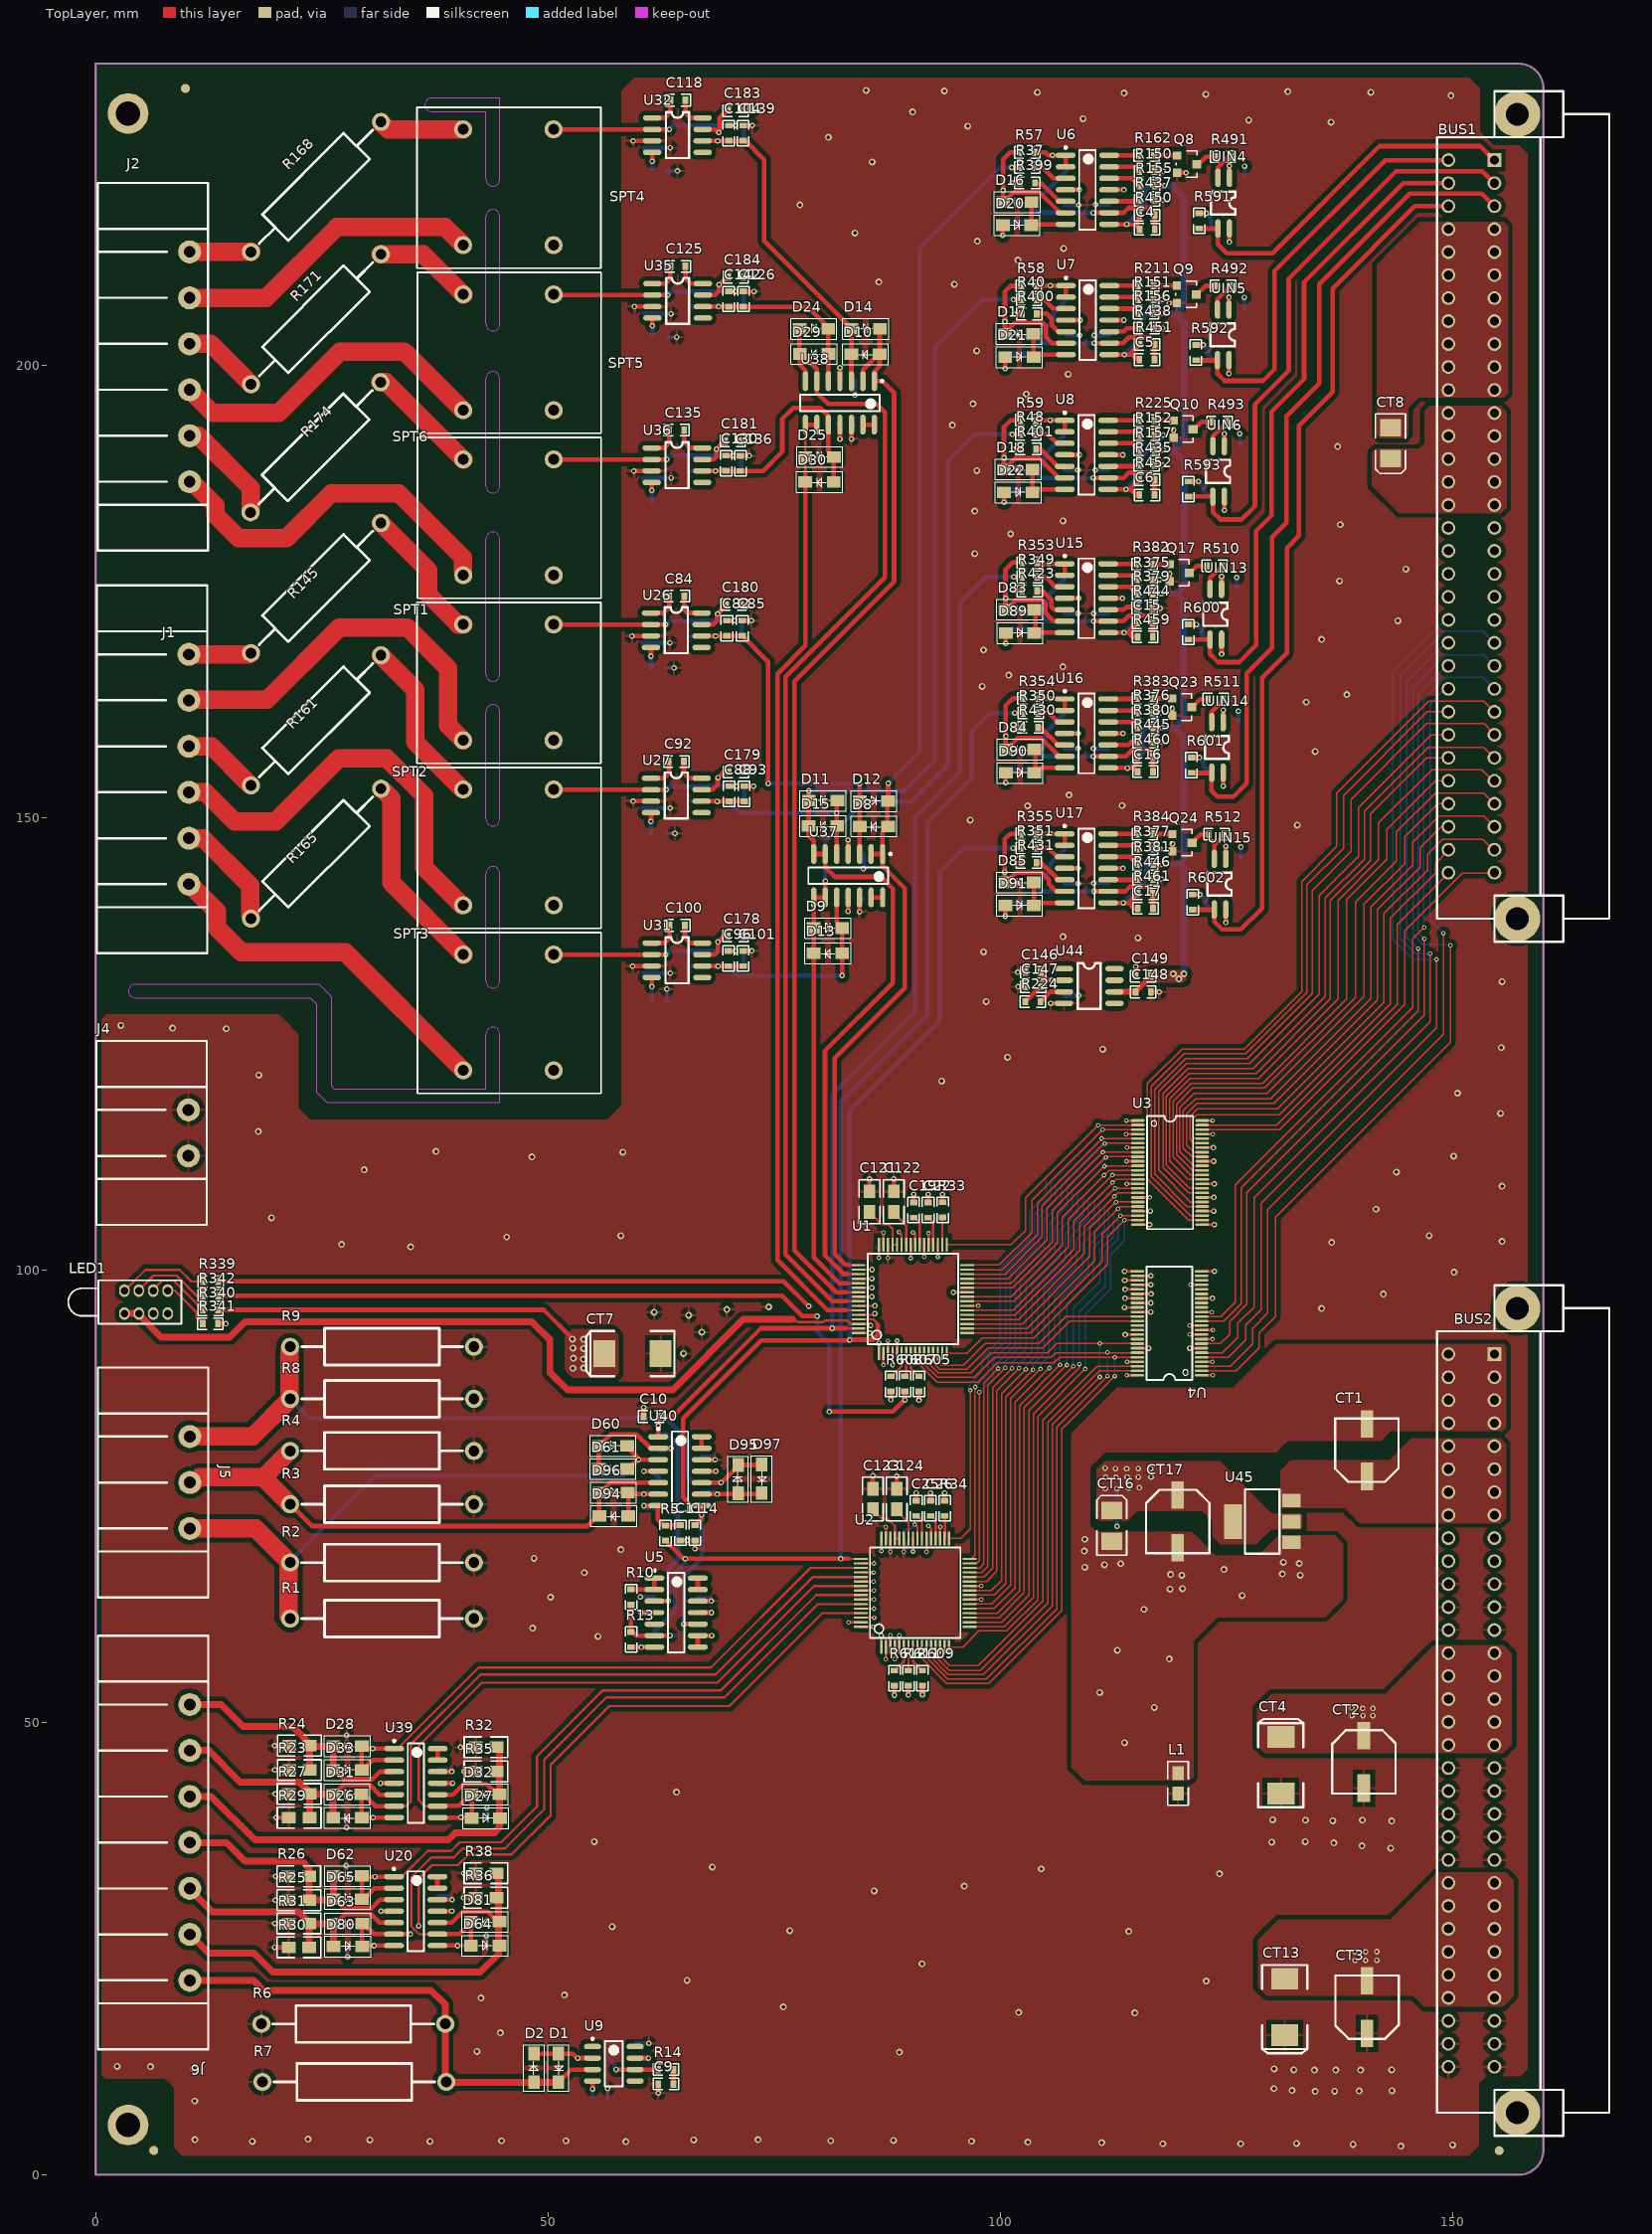
[diagram p0: TopLayer view]
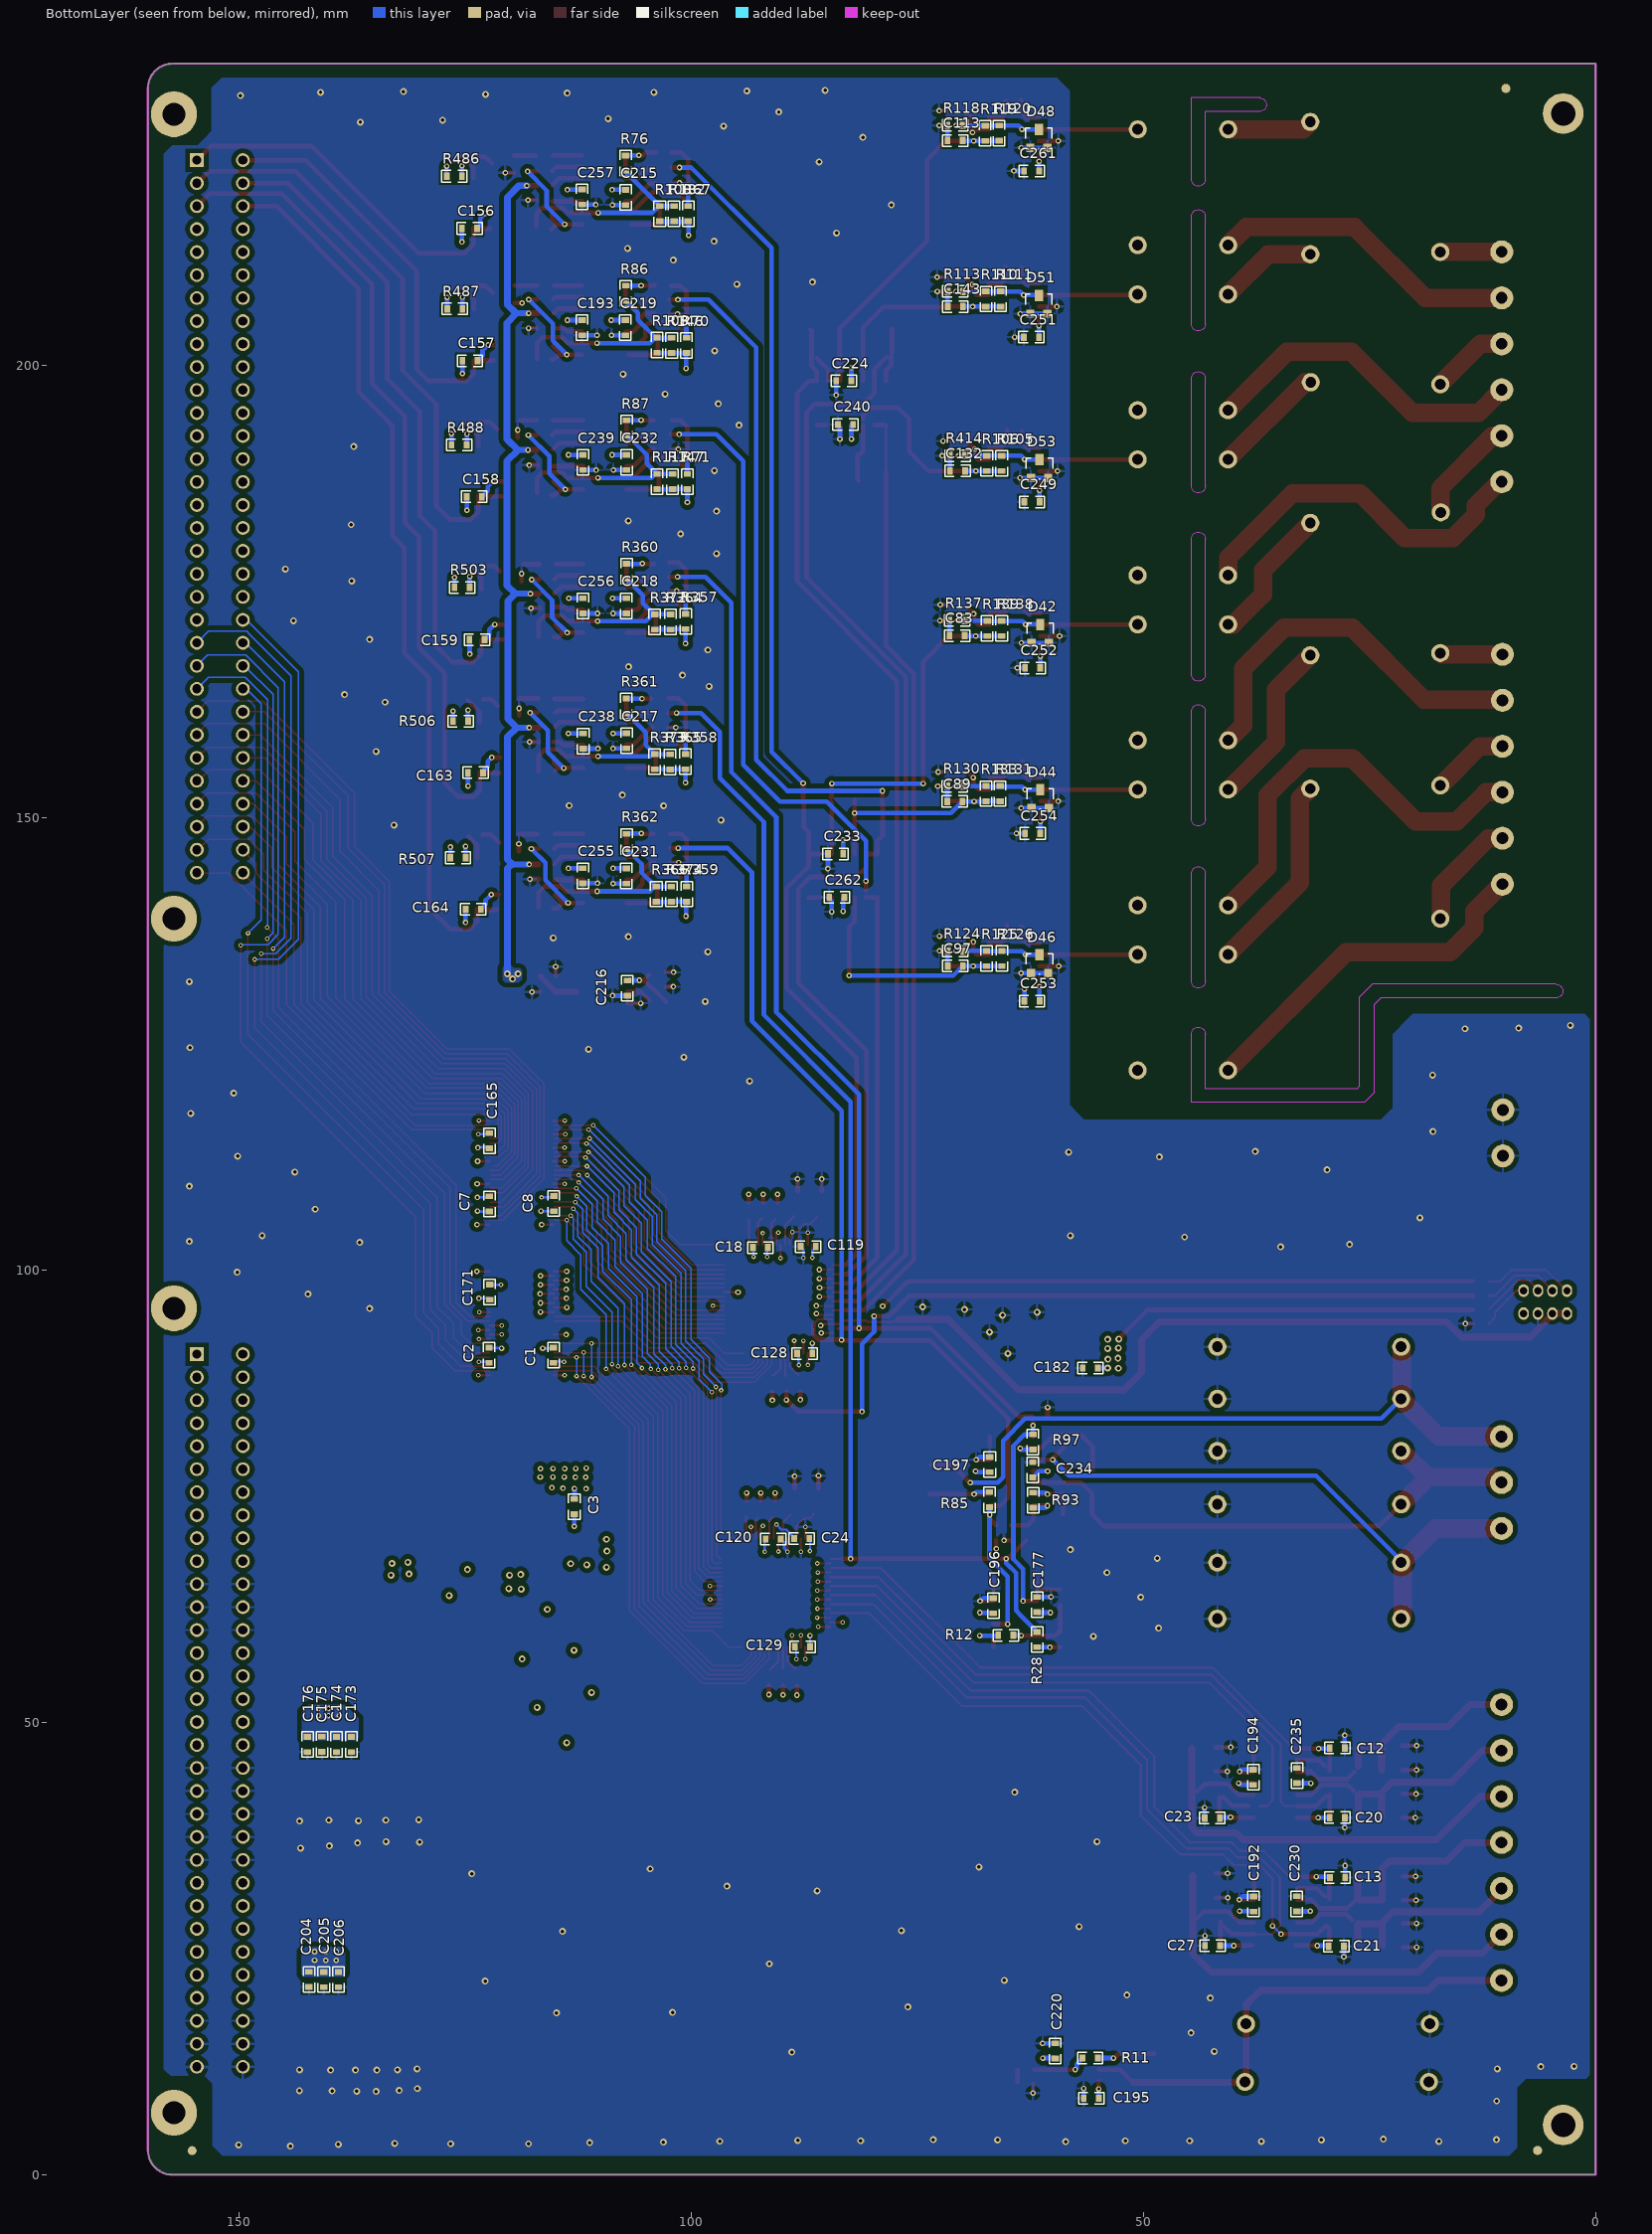
[diagram p1: BottomLayer view, seen from below]
# Altium PCB MISC80584.PCBDoc (part 1 of 7)
Units mm, origin at the board's own origin, x right, y up, seen from the top; angles counter-clockwise.
Board outline 160.02 x 233.3 mm, 4 copper layers (TopLayer, GND, POWER, BottomLayer); 386 components, 266 nets, 1374 pads, 640 vias.

## Layer stack, top to bottom (the 12.6 mil dielectric is the usual default, probably not edited)
TopLayer: signal copper 0.0356
Dielectric: core 0.32, FR-4, Dk 4.8
GND: plane copper 0.0356, net AGND
Dielectric: prepreg 0.32, FR-4, Dk 4.8
POWER: plane copper 0.0356, net (Multiple Nets)
Dielectric: core 0.32, FR-4, Dk 4.8
BottomLayer: signal copper 0.0356

## Board outline
0,0.025 0,233.324 157.302,233.324 cw(c157.302,230.607) 160.02,230.607 160.02,2.743 cw(c157.302,2.743) 157.302,0.025

## Design rules (kind name [scope] priority, off if disabled: settings)
Clearance Clearance_1 [inpolygon{AGND}] p1: gap=0.508
Clearance [All] p2: gap=0.14
FabricationTestPointUsage TestPointUsage [All] p1: valid=0 allowmultiple=FALSE
FabricationTestpoint Testpoint [(IsPad And (OnTopLayer Or OnBottomLayer))] p1: side=3 testpointundercomponent=TRUE minsize=1.016 maxsize=2.54 preferedsize=1.524 minholesize=0.508 maxholesize=1.016 preferedholesize=0.813 testpointgrid=0.025 allowsidetop=TRUE allowsidebottom=TRUE usegrid=TRUE gridtolerance=0
HoleSize [All] p1: absolutevalues=TRUE maxlimit=25.4 minlimit=0.025 maxpercent=80.000 minpercent=20.000
HoleToHoleClearance [All] p1: gap=0 allowstackedmicrovias=TRUE
MinimumSolderMaskSliver [All] p1: minsoldermaskwidth=0
PlaneClearance [All] p1: clearance=0.508
PlaneConnect [All] p1: planeconnectstyle=Direct reliefexpansion=0.508 reliefentries=4 reliefconductorwidth=0.254 reliefairgap=0.254
PolygonConnect PolygonConnect_1 [InNet(AGND)] p1: connectstyle=Relief reliefconductorwidth=0.305 reliefentries=4 polygonreliefangle="90 Angle"
PolygonConnect [All] p2: connectstyle=Direct reliefconductorwidth=0.254 reliefentries=4 polygonreliefangle="90 Angle"
RoutingVias [All] p1: holewidth=0.254 width=0.508 viastyle="Through Hole" minholewidth=0.254 minwidth=0.508 maxholewidth=0.305 maxwidth=0.61
SilkToSilkClearance [All] p1: silktosilkclearance=0
SilkscreenOverComponentPads [All] p1: minsilkscreentomaskgap=0
SolderMaskExpansion [All] p1: expansion=0.102
Width [All] p1: maxlimit=2.54 minlimit=0.152 preferedwidth=0.152 minimp=50.000000 maximp=50.000000 favimp=50.000000
19 further rules are at their usual default settings.

## Components (designator, comment, footprint, x,y, rotation, side; value= is the part's Value field where it differs from the comment)
BUS1 "CON64" BUS64W-A 154.61,222.656 r270 top
BUS2 "CON64" BUS64W-A 154.61,90.703 r270 top
C1 "0.1uF" 0603 115.189,89.764 r90 bottom
C2 "0.1uF" 0603 122.326,91.44 r270 bottom
C3 "0.1uF" 0603 112.903,74.701 r270 bottom
C4 "0.1uF" 0603 115.392,215.011 r0 top
C5 "0.1uF" 0603 115.367,200.609 r0 top
C6 "0.1uF" 0603 115.367,185.649 r0 top
C7 "0.1uF" 0603 122.276,106.477 r90 bottom
C8 "0.1uF" 0603 115.164,108.179 r270 bottom
C9 "0.1uF" 0603 62.205,10.058 r0 top
C10 "30p" 0603 60.579,83.82 r0 top
C11 "30p" 0603 64.618,70.129 r90 top
C12 "30p" 0603 27.737,47.193 r0 bottom
C13 "30p" 0603 27.711,32.868 r0 bottom
C14 "30p" 0603 66.243,70.129 r90 top
C15 "0.1uF" 0603 115.138,171.526 r0 top
C16 "0.1uF" 0603 115.189,155.092 r0 top
C17 "0.1uF" 0603 115.214,139.979 r0 top
C18 "1uF" 0603 91.491,102.489 r0 bottom
C19 "1uF" 0603 90.424,107.467 r270 top
C20 "30p" 0603 27.737,39.497 r0 bottom
C21 "30p" 0603 27.838,25.273 r0 bottom
C22 "1uF" 0603 92.024,107.467 r270 top
C23 "30p" 0603 43.231,39.446 r180 bottom
C24 "1uF" 0603 86.919,70.333 r0 bottom
C25 "1uF" 0603 90.703,74.524 r270 top
C26 "1uF" 0603 92.278,74.524 r270 top
C27 "30p" 0603 43.18,25.349 r180 bottom
C82 "680p" 0603 69.774,170.104 r90 top
C83 "1000p" 0603 69.748,170.104 r0 bottom
C84 "30p" 0603 65.075,174.473 r180 top
C85 "30p" 0603 71.476,171.78 r270 top
C88 "680p" 0603 70.028,151.79 r90 top
C89 "1000p" 0603 70.002,151.79 r0 bottom
C92 "30p" 0603 65.024,156.21 r180 top
C93 "30p" 0603 71.679,153.467 r270 top
C96 "680p" 0603 69.952,133.604 r90 top
C97 "1000p" 0603 69.952,133.604 r0 bottom
C100 "30p" 0603 65.126,138.1 r180 top
C101 "30p" 0603 71.577,135.28 r270 top
C104 "680p" 0603 69.977,224.815 r90 top
C113 "1000p" 0603 69.977,224.815 r0 bottom
C118 "30p" 0603 65.202,229.286 r180 top
C119 "0.1uF" 0603 86.208,102.591 r0 bottom
C120 "0.1uF" 0603 91.745,70.282 r180 bottom
C121 "10u" 0805 85.547,108.712 r270 top
C122 "10u" 0805 88.214,108.712 r270 top
C123 "10u" 0805 85.903,75.844 r270 top
C124 "10u" 0805 88.544,75.844 r270 top
C125 "30p" 0603 65.202,210.922 r180 top
C126 "30p" 0603 71.603,208.153 r270 top
C128 "0.1uF" 0603 86.589,90.78 r0 bottom
C129 "0.1uF" 0603 86.843,58.369 r0 bottom
C130 "680p" 0603 69.672,188.341 r90 top
C132 "1000p" 0603 69.698,188.316 r0 bottom
C135 "30p" 0603 65.049,192.837 r180 top
C136 "30p" 0603 71.272,189.992 r270 top
C139 "30p" 0603 71.577,226.492 r270 top
C142 "680p" 0603 69.977,206.477 r90 top
C143 "1000p" 0603 69.952,206.477 r0 bottom
C146 "1uF" 0603 104.47,132.918 r180 top
C147 "0.1uF" 0603 104.47,131.318 r180 top
C148 "1uF" 0603 114.96,130.734 r0 top
C149 "0.1uF" 0603 114.96,132.486 r0 top
C156 "0.1uF" 0603 123.647,215.113 r0 bottom
C157 "0.1uF" 0603 125.273,200.482 r180 bottom
C158 "0.1uF" 0603 124.79,185.471 r180 bottom
C159 "0.1uF" 0603 122.809,169.672 r0 bottom
C163 "0.1uF" 0603 124.663,154.965 r180 bottom
C164 "0.1uF" 0603 124.917,139.878 r180 bottom
C165 "0.1uF" 0603 122.276,115.138 r270 bottom
C171 "0.1uF" 0603 122.25,96.723 r90 bottom
C173 "0.1uF" 0603 137.541,46.736 r90 bottom
C174 "0.1uF" 0603 139.192,48.412 r270 bottom
C175 "0.1uF" 0603 140.792,48.438 r270 bottom
C176 "0.1uF" 0603 142.392,46.736 r90 bottom
C177 "0.1uF" 0603 61.747,62.205 r90 bottom
C178 "0.1uF" 0603 71.552,136.906 r180 top
C179 "0.1uF" 0603 71.628,155.042 r180 top
C180 "0.1uF" 0603 69.698,173.533 r0 top
C181 "0.1uF" 0603 69.596,191.618 r0 top
C182 "0.1uF" 0603 56.693,89.179 r180 bottom
C183 "0.1uF" 0603 71.577,228.117 r180 top
C184 "0.1uF" 0603 69.926,209.728 r0 top
C192 "0.1uF" 0603 37.821,30.785 r270 bottom
C193 "0.1uF" 0603 112.039,204.978 r270 bottom
C194 "0.1uF" 0603 37.846,44.806 r270 bottom
C195 "0.1uF" 0603 54.915,8.484 r0 bottom
C196 "0.1uF" 0603 66.573,62.078 r90 bottom
C197 "0.1uF" 0603 66.98,79.35 r270 bottom
C204 "0.1uF" 0603 142.215,20.777 r90 bottom
C205 "0.1uF" 0603 140.589,20.752 r90 bottom
C206 "0.1uF" 0603 138.963,22.428 r270 bottom
C215 "0.1uF" 0603 107.213,219.38 r270 bottom
C216 "0.1uF" 0603 107.036,130.327 r90 bottom
C217 "0.1uF" 0603 107.112,157.658 r90 bottom
C218 "0.1uF" 0603 107.137,174.244 r270 bottom
C219 "0.1uF" 0603 107.264,203.302 r90 bottom
C220 "0.1uF" 0603 59.741,14.554 r270 bottom
C224 "0.1uF" 0603 82.271,198.272 r0 bottom
C230 "0.1uF" 0603 33.045,30.81 r270 bottom
C231 "0.1uF" 0603 107.137,144.399 r270 bottom
C232 "0.1uF" 0603 107.112,190.094 r270 bottom
C233 "0.1uF" 0603 84.861,145.999 r180 bottom
C234 "0.1uF" 0603 62.23,77.089 r90 bottom
C235 "0.1uF" 0603 33.02,44.983 r270 bottom
C238 "0.1uF" 0603 111.912,157.632 r90 bottom
C239 "0.1uF" 0603 111.938,190.094 r270 bottom
C240 "0.1uF" 0603 82.093,193.446 r0 bottom
C249 "0.1uF" 0603 61.468,184.887 r0 bottom
C251 "0.1uF" 0603 63.221,203.098 r180 bottom
C252 "0.1uF" 0603 61.392,166.548 r0 bottom
C253 "0.1uF" 0603 63.144,129.743 r180 bottom
C254 "0.1uF" 0603 61.392,148.26 r0 bottom
C255 "0.1uF" 0603 111.963,144.424 r270 bottom
C256 "0.1uF" 0603 111.938,172.568 r90 bottom
C257 "0.1uF" 0603 112.039,217.754 r90 bottom
C261 "0.1uF" 0603 63.195,221.463 r180 bottom
C262 "0.1uF" 0603 83.033,141.199 r0 bottom
CT1 "100uF/16V" L470UF 140.513,82.753 r180 top
CT2 "100uF/35V" L470UF 140.183,43.002 r0 top
CT3 "100uF/35V" L470UF 140.538,21.209 r180 top
CT4 "22u/35V" 7343_CASE-D 131.013,45.288 r90 top
CT7 "22u/35V" 7343_CASE-D 59.334,90.78 r180 top
CT8 "22u/16V" 3528_CASE-B 143.129,189.662 r90 top
CT13 "22u/35V" 7343_CASE-D 131.445,18.567 r270 top
CT16 "22u/16V" 3528_CASE-B 112.319,73.457 r270 top
CT17 "100uF/16V" L470UF 119.609,69.571 r0 top
D1 "1N4148" 1N4148-A 51.156,13.411 r270 top
D2 "1N4148" 1N4148-A 48.463,10.262 r90 top
D8 "1N4148" 1N4148-A 87.605,149.047 r180 top
D9 "1N4148" 1N4148-A 79.375,137.795 r0 top
D10 "1N4148" 1N4148-A 86.665,201.219 r180 top
D11 "1N4148" 1N4148-A 78.842,151.867 r0 top
D12 "1N4148" 1N4148-A 84.455,151.841 r0 top
D13 "1N4148" 1N4148-A 82.525,135.026 r180 top
D14 "1N4148" 1N4148-A 83.541,204.013 r0 top
D15 "1N4148" 1N4148-A 81.966,149.098 r180 top
D16 "1N4148" 1N4148-A 103.454,218.034 r180 top
D17 "1N4148" 1N4148-A 103.657,203.479 r180 top
D18 "1N4148" 1N4148-A 103.556,188.493 r180 top
D20 "1N4148" 1N4148-A 100.279,215.468 r0 top
D21 "1N4148" 1N4148-A 100.533,200.889 r0 top
D22 "1N4148" 1N4148-A 100.406,185.953 r0 top
D24 "1N4148" 1N4148-A 77.826,204.013 r0 top
D25 "1N4148" 1N4148-A 78.461,189.865 r0 top
D26 "1N4148" 1N4148-A 29.413,39.497 r180 top
D27 "1N4148" 1N4148-A 41.554,39.446 r0 top
D28 "1N4148" 1N4148-A 29.413,47.396 r180 top
D29 "1N4148" 1N4148-A 81.001,201.244 r180 top
D30 "1N4148" 1N4148-A 81.585,187.096 r180 top
D31 "1N4148" 1N4148-A 26.238,42.062 r0 top
D32 "1N4148" 1N4148-A 44.653,42.062 r180 top
D33 "1N4148" 1N4148-A 26.264,44.78 r0 top
D42 "BAV99W" SOT23R 62.357,169.316 r180 bottom
D44 "BAV99W" SOT23R 62.357,151.054 r180 bottom
D46 "BAV99W" SOT23R 62.433,132.817 r180 bottom
D48 "BAV99W" SOT23R 62.509,224.028 r180 bottom
D51 "BAV99W" SOT23R 62.509,205.689 r180 bottom
D53 "BAV99W" SOT23R 62.433,187.554 r180 bottom
D60 "1N4148" 1N4148-A 55.626,80.594 r0 top
D61 "1N4148" 1N4148-A 58.776,78.029 r180 top
D62 "1N4148" 1N4148-A 29.439,33.045 r180 top
D63 "1N4148" 1N4148-A 29.464,27.788 r180 top
D64 "1N4148" 1N4148-A 41.478,25.349 r0 top
D65 "1N4148" 1N4148-A 26.289,30.505 r0 top
D80 "1N4148" 1N4148-A 26.314,25.273 r0 top
D81 "1N4148" 1N4148-A 44.628,27.991 r180 top
D83 "1N4148" 1N4148-A 103.734,172.999 r180 top
D84 "1N4148" 1N4148-A 103.759,157.531 r180 top
D85 "1N4148" 1N4148-A 103.708,142.85 r180 top
D89 "1N4148" 1N4148-A 100.609,170.409 r0 top
D90 "1N4148" 1N4148-A 100.609,154.94 r0 top
D91 "1N4148" 1N4148-A 100.559,140.284 r0 top
D94 "1N4148" 1N4148-A 58.852,72.847 r180 top
D95 "1N4148" 1N4148-A 71.018,75.336 r90 top
D96 "1N4148" 1N4148-A 55.677,75.413 r0 top
D97 "1N4148" 1N4148-A 73.635,78.511 r270 top
J1 "CON6" EDGCon_6P_5.08mm_ear 10.312,168.046 r270 top
J2 "CON6" EDGCon_6P_5.08mm_ear 10.389,212.522 r270 top
J4 "Header2" EDGCON_2p_5.08mm_ear 10.262,112.624 r270 top
J5 "Header3" EDGCON_3p_5.08mm_ear 10.414,76.53 r270 top
J6 "Header7" EDGCon_7P_5.08mm_ear 10.414,51.994 r270 top
L1 "1uH" 0805 119.634,44.425 r270 top
LED1 "LEDGroup_4" LEDGroup_4 3.175,95.199 r0 top
Q8 "2N2222" SOT23-3 121.717,219.989 r270 top
Q9 "2N2222" SOT23-3 121.666,205.613 r270 top
Q10 "2N2222" SOT23-3 121.31,190.703 r270 top
Q17 "2N2222" SOT23-3 120.879,174.828 r270 top
Q23 "2N2222" SOT23-3 121.158,159.995 r270 top
Q24 "2N2222" SOT23-3 121.183,145.009 r270 top
R1 "100Ω_2W_1%" AXIAL0.8 41.808,61.468 r180 top
R2 "100Ω_2W_1%" AXIAL0.8 41.808,67.666 r180 top
R3 "100Ω_2W_1%" AXIAL0.8 41.808,74.117 r180 top
R4 "100Ω_2W_1%" AXIAL0.8 41.808,80.01 r180 top
R5 "0" 0603 62.992,70.104 r90 top
R6 "2W_1%" AXIAL0.8 18.339,16.713 r0 top
R7 "2W_1%" AXIAL0.8 18.449,10.299 r0 top
R8 "100Ω_2W_1%" AXIAL0.8 41.808,85.764 r180 top
R9 "100Ω_2W_1%" AXIAL0.8 41.808,91.516 r180 top
R10 "10k_1%" 0603 59.182,63.043 r90 top
R11 "4.7k" 0603 56.718,12.929 r180 bottom
R12 "10k_1%" 0603 64.364,59.639 r0 bottom
R13 "10k_1%" 0603 59.182,58.344 r90 top
R14 "10k" 0603 63.881,11.659 r180 top
R23 "2k" 0805 23.673,44.755 r180 top
R24 "2k" 0805 23.673,47.447 r180 top
R25 "2k" 0805 23.622,30.378 r180 top
R26 "2k" 0805 23.597,33.02 r180 top
R27 "2k" 0805 23.647,42.113 r180 top
R28 "0" 0603 61.747,60.02 r270 bottom
R29 "2k" 0805 23.647,39.497 r180 top
R30 "2k" 0805 23.622,25.171 r180 top
R31 "2k" 0805 23.622,27.813 r180 top
R32 "2k" 0805 44.298,47.269 r180 top
R33 "10k" 0603 93.624,105.816 r90 top
R34 "10k" 0603 93.853,72.847 r90 top
R35 "2k" 0805 44.298,44.602 r180 top
R36 "2k" 0805 44.298,30.658 r180 top
R37 "10k" 0603 103.835,221.844 r180 top
R38 "2k" 0805 44.298,33.35 r180 top
R40 "10k" 0603 104.013,207.239 r180 top
R48 "10k" 0603 103.911,192.354 r180 top
R57 "10k" 0603 102.133,223.52 r0 top
R58 "10k" 0603 102.311,208.788 r0 top
R59 "10k" 0603 102.235,193.929 r0 top
R67 "10k" 0603 100.305,215.9 r90 bottom
R70 "10k" 0603 100.508,201.346 r90 bottom
R71 "10k" 0603 100.406,186.309 r90 bottom
R76 "10k" 0603 107.239,221.488 r90 bottom
R85 "4.7k" 0603 67.005,73.787 r90 bottom
R86 "10k" 0603 107.213,207.112 r90 bottom
R87 "10k" 0603 107.112,192.227 r90 bottom
R93 "4.7k" 0603 62.179,73.736 r90 bottom
R97 "4.7k" 0603 62.205,81.839 r270 bottom
R100 "10k" 0603 103.454,217.576 r270 bottom
R105 "5.1k_1%" 0603 65.659,188.316 r90 bottom
R106 "5.1k_1%" 0603 67.31,188.316 r90 bottom
R108 "10k" 0603 103.759,203.048 r270 bottom
R110 "5.1k_1%" 0603 67.412,206.477 r90 bottom